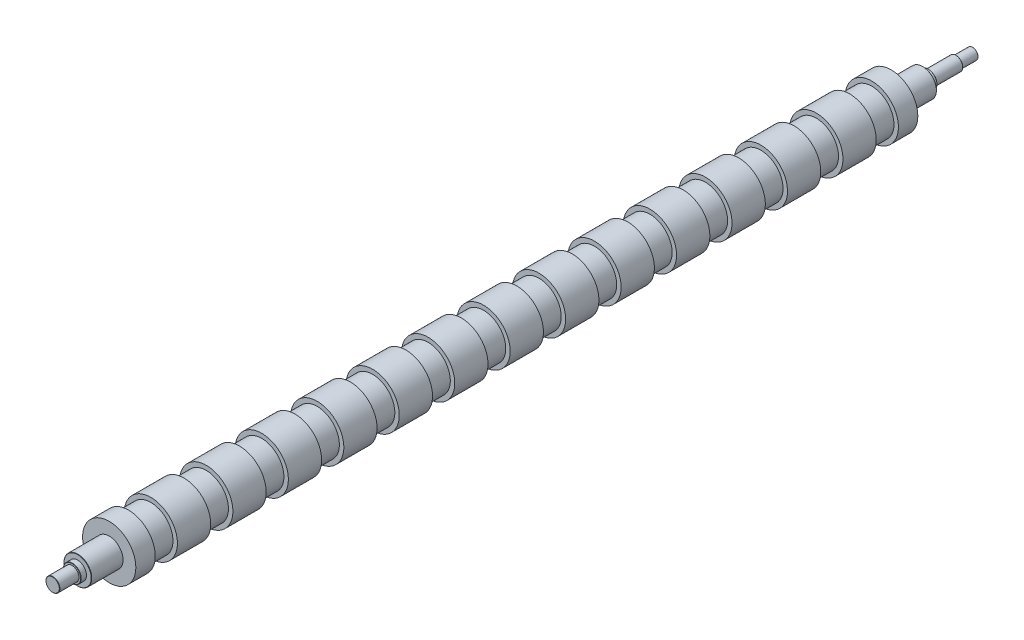
from build123d import *

# Parameters (mm, degrees)
SKETCH_1_R             = 48
EXTRUDE_1_DEPTH        = 1410
SKETCH_2_R             = 16
EXTRUDE_2_DEPTH        = 67
EXTRUDE_START          = 67
SKETCH_3_R             = 16
EXTRUDE_3_DEPTH        = 67
SKETCH_4_R             = 12.5
EXTRUDE_4_DEPTH        = 80
EXTRUDE_START_2        = 35
SKETCH_5_R             = 12.5
EXTRUDE_5_DEPTH        = 35
SKETCH_6_OUTSIDE_W     = 430.91
SKETCH_6_OUTSIDE_H     = 430.91
SKETCH_6_OUTSIDE_R     = 10
CUT_EXTRUDE_1_DEPTH    = 30
SKETCH_7_W             = 40
SKETCH_7_H             = 8
PATTERN_LINEAR_1_COUNT = 14
PATTERN_LINEAR_1_PITCH = 100
SKETCH_9_R             = 25
EXTRUDE_6_DEPTH        = 57
EXTRUDE_START_3        = 57
SKETCH_10_R            = 25
EXTRUDE_7_DEPTH        = 57
CHAMFER_1_SIZE         = 0.5


with BuildPart() as part:
    # 草图1 → 凸台-拉伸1 (new body)
    with BuildSketch(Plane.XY):
        Circle(SKETCH_1_R)
    extrude(amount=EXTRUDE_1_DEPTH)

    # 草图2 → 凸台-拉伸2 (add)
    with BuildSketch(Plane.XY.offset(1410)):
        Circle(SKETCH_2_R)
    extrude(amount=EXTRUDE_2_DEPTH)

    # 草图3 → 凸台-拉伸3 (add)
    with BuildSketch(Plane(origin=(0, 0, 0), x_dir=(-1, 0, 0), z_dir=(0, 0, -1)).offset(EXTRUDE_START)):
        with Locations(Location((0, 0, 0), (0, 0, 180))):
            Circle(SKETCH_3_R)
    extrude(amount=-EXTRUDE_3_DEPTH)

    # 草图4 → 凸台-拉伸4 (add)
    with BuildSketch(Plane(origin=(0, 0, -67), x_dir=(-1, 0, 0), z_dir=(0, 0, -1))):
        Circle(SKETCH_4_R)
    extrude(amount=EXTRUDE_4_DEPTH)

    # 草图5 → 凸台-拉伸5 (add)
    with BuildSketch(Plane.XY.offset(1477).offset(EXTRUDE_START_2)):
        with Locations(Location((0, 0, 0), (0, 0, 180))):
            Circle(SKETCH_5_R)
    extrude(amount=-EXTRUDE_5_DEPTH)

    # 草图6 outside → 切除-拉伸1 (cut)
    with BuildSketch(Plane(origin=(0, 0, -147), x_dir=(-1, 0, 0), z_dir=(0, 0, -1))):
        Rectangle(SKETCH_6_OUTSIDE_W, SKETCH_6_OUTSIDE_H)
        Circle(SKETCH_6_OUTSIDE_R, mode=Mode.SUBTRACT)
    extrude(amount=-CUT_EXTRUDE_1_DEPTH, mode=Mode.SUBTRACT)

    # 草图7 → 切除-旋转1 (revolve, cut)
    with BuildSketch(Plane(origin=(0, 0, 0), x_dir=(0, 0, -1), z_dir=(1, 0, 0)), mode=Mode.PRIVATE) as cut_revolve_1_sk:
        with Locations((-55, -44)):
            Rectangle(SKETCH_7_W, SKETCH_7_H)
    cut_revolve_1 = revolve(cut_revolve_1_sk.sketch.rotate(Axis((0, 0, 0), (0, 0, 1)), 270), axis=Axis((0, 0, 0), (0, 0, 1)), mode=Mode.SUBTRACT)

    # 阵列(线性)1: 切除-旋转1 ×14
    with Locations(*[(0, 0, i * PATTERN_LINEAR_1_PITCH) for i in range(1, PATTERN_LINEAR_1_COUNT)]):
        add(cut_revolve_1, mode=Mode.SUBTRACT)

    # 草图9 → 凸台-拉伸6 (add)
    with BuildSketch(Plane.XY.offset(1410)):
        with Locations(Location((0, 0, 0), (0, 0, 180))):
            Circle(SKETCH_9_R)
    extrude(amount=EXTRUDE_6_DEPTH)

    # 草图10 → 凸台-拉伸7 (add)
    with BuildSketch(Plane(origin=(0, 0, 0), x_dir=(-1, 0, 0), z_dir=(0, 0, -1)).offset(EXTRUDE_START_3)):
        Circle(SKETCH_10_R)
    extrude(amount=-EXTRUDE_7_DEPTH)

    # 倒角1
    chamfer_1_edges = [part.edges().sort_by_distance(p)[0] for p in [
        (-16, 0, -67),
        (25, 0, 1467),
        (25, 0, -57),
        (12.5, 0, 1512),
        (12.5, 0, -117),
        (10, 0, -147),
        (-16, 0, 1477),
    ]]
    chamfer(chamfer_1_edges, length=CHAMFER_1_SIZE)


solid = part.part
